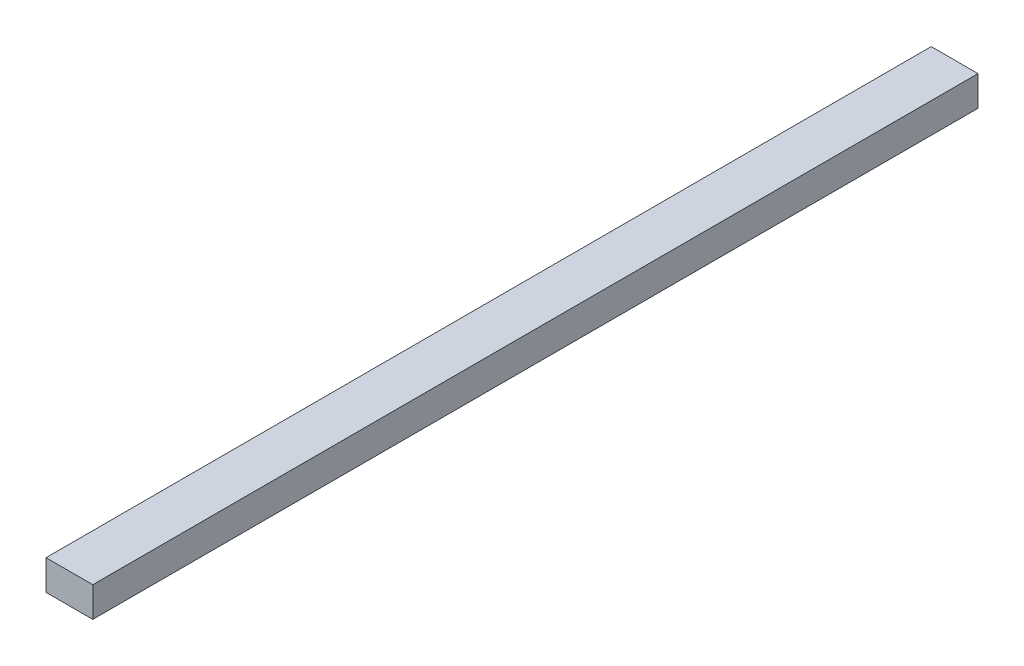
SolidWorks part; units mm, degrees
ref_plane "Front Plane" through (0, 0, 0) normal (0, 0, 1) x (1, 0, 0)
ref_plane "Top Plane" through (0, 0, 0) normal (0, 1, 0) x (1, 0, 0)
ref_plane "Right Plane" through (0, 0, 0) normal (1, 0, 0) x (0, 0, -1)
ref_plane "Plane1" through (0, 164.944, 0) normal (0, 1, 0) x (1, 0, 0)
sketch "Sketch1" plane through (0, 164.944, 0) normal (0, 1, 0) x (1, 0, 0)
  line L0 (514.2306, 660.693) -> (528.2306, 660.693)
  line L1 (528.2306, 660.693) -> (528.2306, 925.693)
  line L2 (528.2306, 925.693) -> (514.2306, 925.693)
  line L3 (514.2306, 925.693) -> (514.2306, 660.693)
  dimension "D1" = 14
  dimension "D2" = 265
extrude "Boss-Extrude1" add sketch "Sketch1" against normal blind 9
